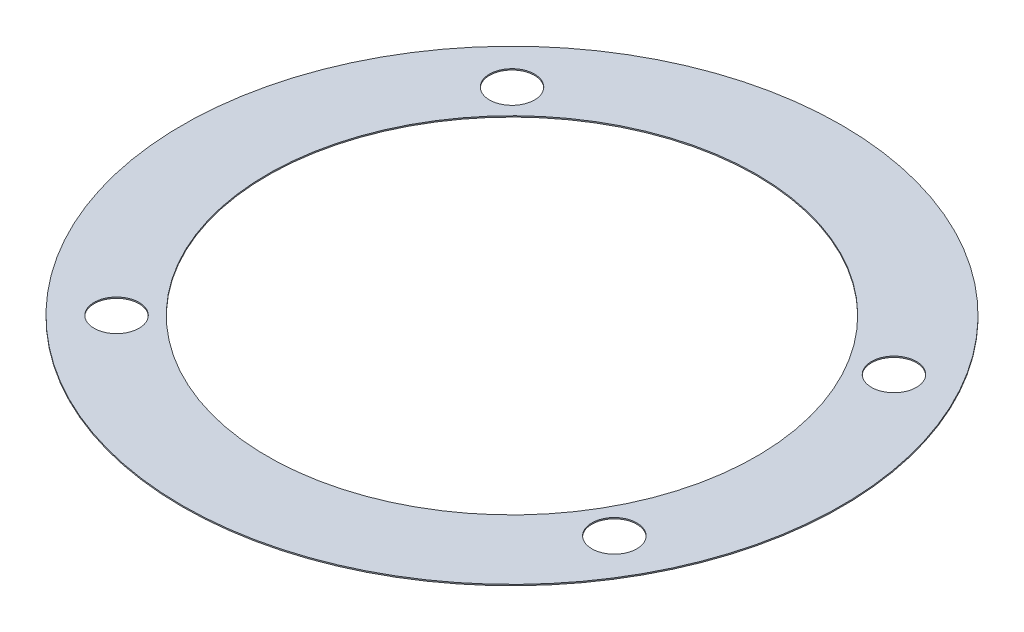
SolidWorks part; units mm, degrees
material "瓦楞纸"
ref_plane "Front Plane" through (0, 0, 0) normal (0, 0, 1) x (1, 0, 0)
ref_plane "Top Plane" through (0, 0, 0) normal (0, 1, 0) x (1, 0, 0)
ref_plane "Right Plane" through (0, 0, 0) normal (1, 0, 0) x (0, 0, -1)
sketch "Sketch1" plane through (0, 0, 0) normal (0, 1, 0) x (1, 0, 0)
  circle A0 centre (0, 0) radius 104.775
  circle A1 centre (0, 0) radius 77.724
  dimension "D1" = 209.55
  dimension "D2" = 155.448
extrude "Boss-Extrude1" add sketch "Sketch1" along normal blind 0.381
hole_wizard "9/16 (0.5625) Diameter Hole1" positions "3DSketch1" profile "Sketch2" hole size "9/16" standard "Ansi Inch"
sketch3d "3DSketch1"
  point P0 (-62.8586, 0.381, -62.865)
  point P2 (76.9874, 0.381, -44.45)
  dimension "D1" = 62.865
  dimension "D2" = 62.8586
  dimension "D3" = 76.9874
  dimension "D4" = 44.45
sketch "Sketch2" plane through (-62.8586, 0.381, -62.865) normal (1, 0, 0) x (0, 0, 1)
  line L0 (0, 0) -> (0, 20.1724)
  line L1 (0, 20.1724) -> (7.1437, 15.88)
  line L2 (7.1437, 15.88) -> (7.1437, 0)
  line L5 (7.1437, 0) -> (0, 0)
  line L10 (0, 20.1724) -> (-7.1437, 15.88) construction
  line L11 (0, -6.35) -> (0, 107.95) construction
  dimension "孔直径" = 14.2875
  dimension "孔深度" = 15.88
  dimension "导头角度" = 118
mirror "Mirror1" about plane through (0, 0, 0) normal (0, 0, 1) of "9/16 (0.5625) Diameter Hole1"
